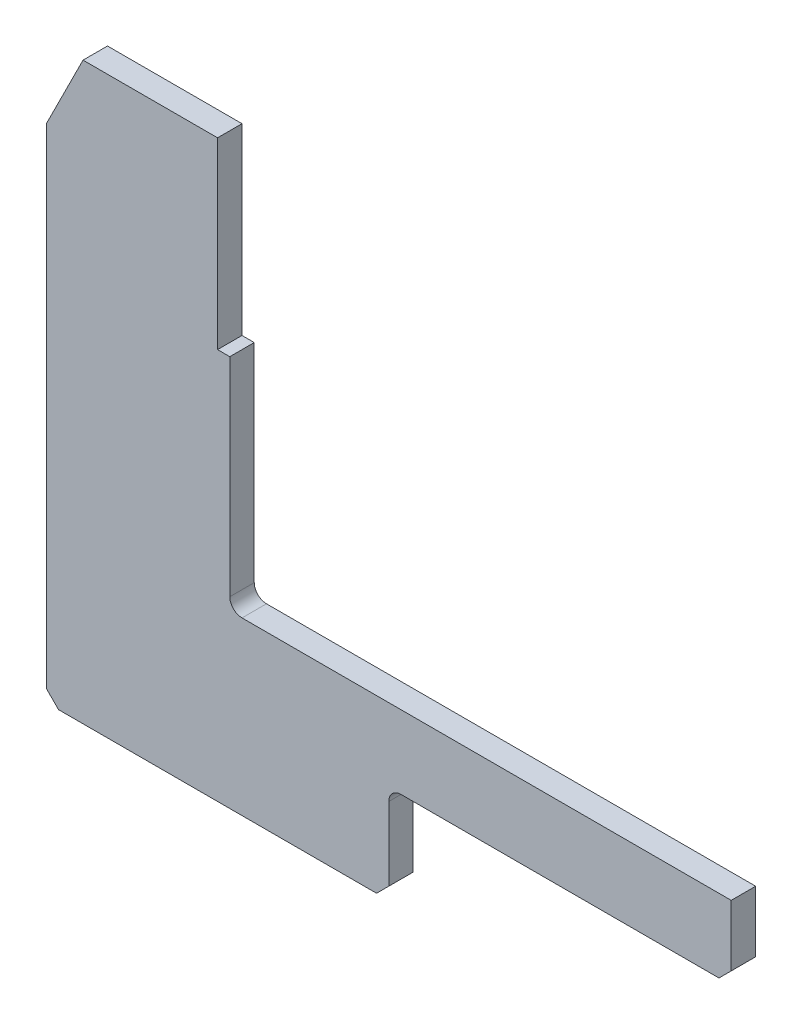
SolidWorks part; units mm, degrees
ref_plane "Front Plane" through (0, 0, 0) normal (0, 0, 1) x (1, 0, 0)
ref_plane "Top Plane" through (0, 0, 0) normal (0, 1, 0) x (1, 0, 0)
ref_plane "Right Plane" through (0, 0, 0) normal (1, 0, 0) x (0, 0, -1)
sketch "Sketch1" plane through (0, 0, 0) normal (0, 0, 1) x (1, 0, 0)
  line L0 (-61.6308, 752.7298) -> (-61.6308, -67.2702)
  line L1 (-61.6308, -67.2702) -> (498.3692, -67.2702)
  line L2 (498.3692, -67.2702) -> (498.3692, 92.7298)
  line L3 (498.3692, 92.7298) -> (1058.3692, 92.7298)
  line L4 (1058.3692, 92.7298) -> (1058.3692, 212.7298)
  line L5 (1058.3692, 212.7298) -> (238.3692, 212.7298)
  line L6 (238.3692, 212.7298) -> (238.3692, 572.7298)
  line L7 (238.3692, 572.7298) -> (218.3692, 572.7298)
  line L8 (218.3692, 572.7298) -> (218.3692, 872.7298)
  line L9 (218.3692, 872.7298) -> (-1.6308, 872.7298)
  line L12 (-61.6308, 752.7298) -> (-1.6308, 872.7298)
extrude "Boss-Extrude1" add sketch "Sketch1" along normal blind 40
chamfer "Chamfer1" distance 20 angle 45 3 edges at (-61.6308, -67.2702, 20) (1058.3692, 92.7298, 20) (498.3692, -67.2702, 20)
fillet "Fillet1" radius 20 2 edges at (498.3692, 92.7298, 20) (238.3692, 212.7298, 20)
